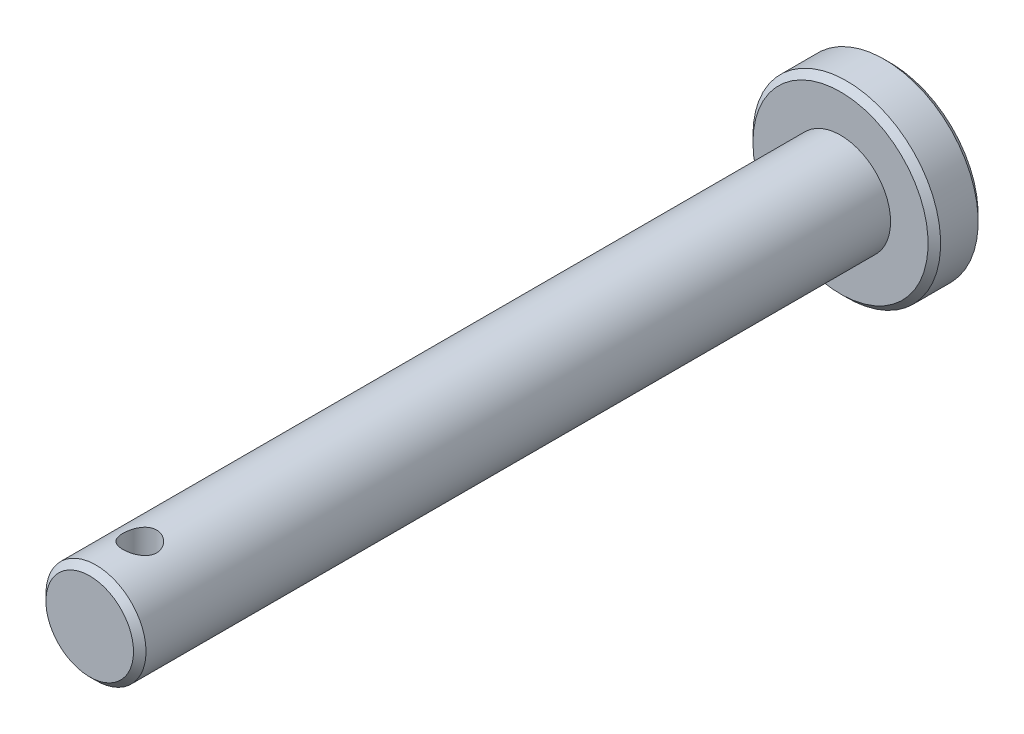
SolidWorks part; units mm, degrees
material "国产6061 "
ref_plane "Front Plane" through (0, 0, 0) normal (0, 0, 1) x (1, 0, 0)
ref_plane "Top Plane" through (0, 0, 0) normal (0, 1, 0) x (1, 0, 0)
ref_plane "Right Plane" through (0, 0, 0) normal (1, 0, 0) x (0, 0, -1)
sketch "Sketch1" plane through (0, 0, 0) normal (0, 0, 1) x (1, 0, 0)
  circle A0 centre (0, 0) radius 4
  dimension "D1" = 8
extrude "Boss-Extrude1" add sketch "Sketch1" along normal blind 60
sketch "Sketch2" plane through (0, 0, 0) normal (0, 0, -1) x (-1, 0, 0)
  circle A0 centre (0, 0) radius 7.5
  dimension "D1" = 15
extrude "Boss-Extrude2" add sketch "Sketch2" along normal blind 4
sketch "Sketch3" plane through (0, 0, 0) normal (0, 1, 0) x (1, 0, 0)
  line L0 (-4, -60) -> (4, -60) construction
  circle A0 centre (0, -56) radius 1.35
  dimension "D1" = 2.7
  dimension "D2" = 4
extrude "Cut-Extrude1" cut sketch "Sketch3" against normal through all both and the other way through all
chamfer "Chamfer1" distance 0.5 angle 45 3 edges at (4, 0, 60) (-7.5, 0, -4) (-7.5, 0, 0)
